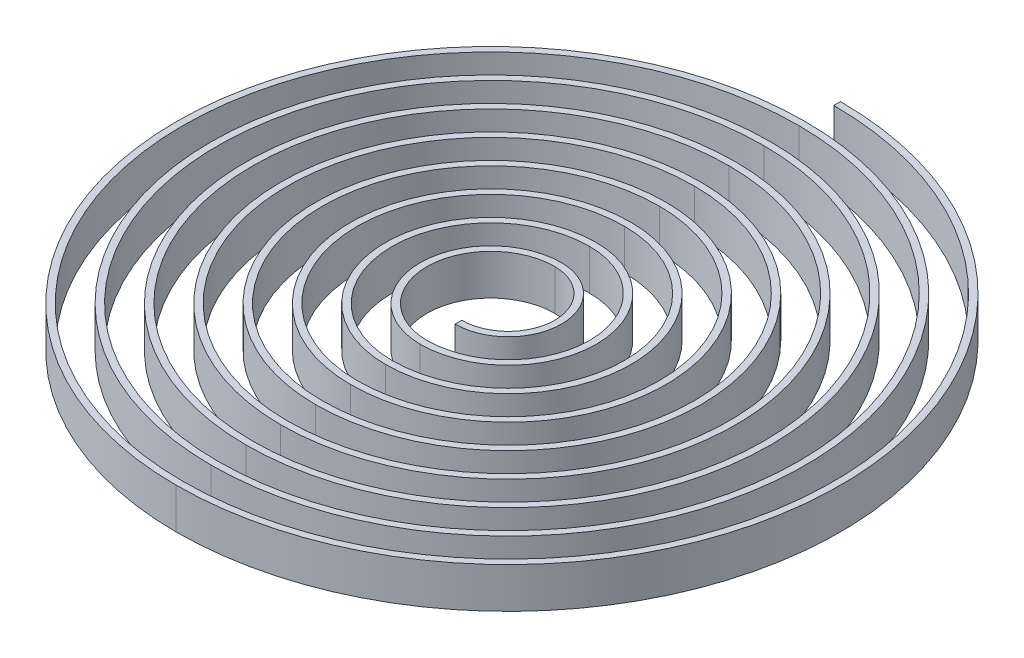
from build123d import *

# Parameters (mm, degrees)
EXTRUDE_THIN_2_DEPTH = 2.18


with BuildPart() as part:
    # Sketch 1 → Extrude-thin 2 (new body)
    with BuildSketch(Plane(origin=(0, 0, 0), x_dir=(1, 0, 0), z_dir=(0, 1, 0))):
        with BuildLine():
            ThreePointArc((0, -2.5), (2.5, 0), (0, 2.5))
            ThreePointArc((0, 2.5), (-3.4375, -0.9375), (0, -4.375))
            ThreePointArc((0, -4.375), (4.375, 0), (0, 4.375))
            ThreePointArc((0, 4.375), (-5.3125, -0.9375), (0, -6.25))
            ThreePointArc((0, -6.25), (6.25, 0), (0, 6.25))
            ThreePointArc((0, 6.25), (-7.1875, -0.9375), (0, -8.125))
            ThreePointArc((0, -8.125), (8.125, 0), (0, 8.125))
            ThreePointArc((0, 8.125), (-9.0625, -0.9375), (0, -10))
            ThreePointArc((0, -10), (10, 0), (0, 10))
            ThreePointArc((0, 10), (-10.9375, -0.9375), (0, -11.875))
            ThreePointArc((0, -11.875), (11.875, 0), (0, 11.875))
            ThreePointArc((0, 11.875), (-12.8125, -0.9375), (0, -13.75))
            ThreePointArc((0, -13.75), (13.75, 0), (0, 13.75))
            ThreePointArc((0, 13.75), (-14.6875, -0.9375), (0, -15.625))
            ThreePointArc((0, -15.625), (15.625, 0), (0, 15.625))
            ThreePointArc((0, 15.625), (-16.5625, -0.9375), (0, -17.5))
            ThreePointArc((0, -17.5), (17.5, 0), (0, 17.5))
            Line((0, 17.5), (0, 17.86))
            ThreePointArc((0, 17.86), (17.86, 0), (0, -17.86))
            ThreePointArc((0, -17.86), (-16.9225, -0.9375), (0, 15.985))
            ThreePointArc((0, 15.985), (15.985, 0), (0, -15.985))
            ThreePointArc((0, -15.985), (-15.0475, -0.9375), (0, 14.11))
            ThreePointArc((0, 14.11), (14.11, 0), (0, -14.11))
            ThreePointArc((0, -14.11), (-13.1725, -0.9375), (0, 12.235))
            ThreePointArc((0, 12.235), (12.235, 0), (0, -12.235))
            ThreePointArc((0, -12.235), (-11.2975, -0.9375), (0, 10.36))
            ThreePointArc((0, 10.36), (10.36, 0), (0, -10.36))
            ThreePointArc((0, -10.36), (-9.4225, -0.9375), (0, 8.485))
            ThreePointArc((0, 8.485), (8.485, 0), (0, -8.485))
            ThreePointArc((0, -8.485), (-7.5475, -0.9375), (0, 6.61))
            ThreePointArc((0, 6.61), (6.61, 0), (0, -6.61))
            ThreePointArc((0, -6.61), (-5.6725, -0.9375), (0, 4.735))
            ThreePointArc((0, 4.735), (4.735, 0), (0, -4.735))
            ThreePointArc((0, -4.735), (-3.7975, -0.9375), (0, 2.86))
            ThreePointArc((0, 2.86), (2.86, 0), (0, -2.86))
            Line((0, -2.86), (0, -2.5))
        make_face()
    extrude(amount=EXTRUDE_THIN_2_DEPTH)


solid = part.part
